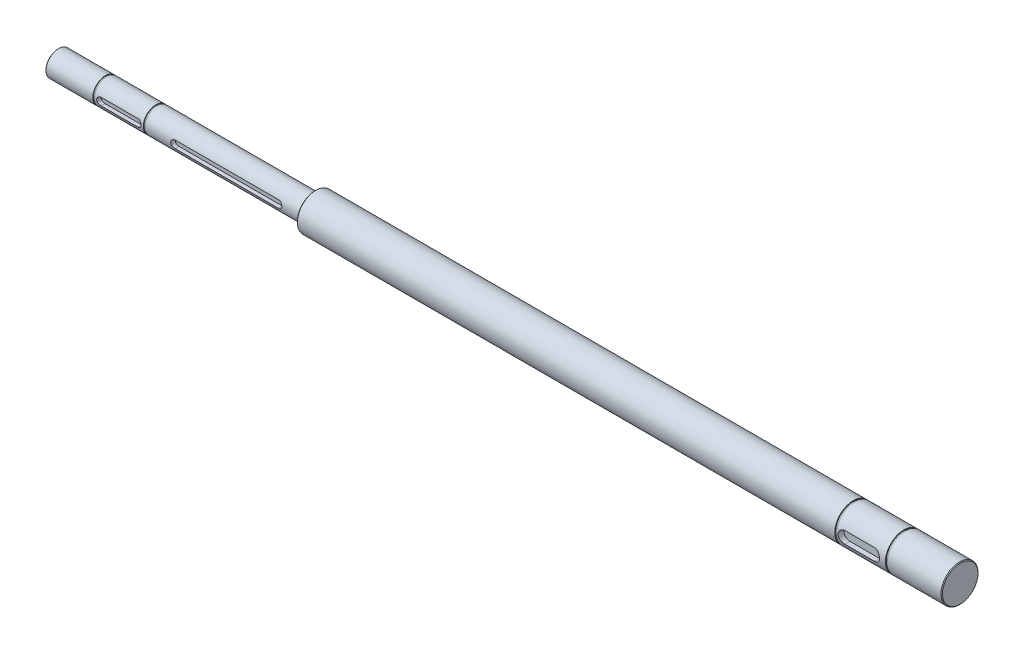
from build123d import *

# Parameters (mm, degrees)
SKETCH_2_R             = 12.5
EXTRUDE_1_DEPTH        = 304.5
SKETCH_3_OUTSIDE_W     = 149.006
SKETCH_3_OUTSIDE_H     = 149.006
SKETCH_3_OUTSIDE_R     = 8.5
CUT_EXTRUDE_1_DEPTH    = 173.5
CUT_EXTRUDE_2_DEPTH    = 3
CUT_EXTRUDE_3_DEPTH    = 4
CHAMFER_1_SIZE         = 0.5
CHAMFER_2_SIZE         = 0.3
SKETCH_8_W             = 1.2
SKETCH_8_H             = 0.55
PATTERN_LINEAR_2_COUNT = 2
PATTERN_LINEAR_2_PITCH = 34.2
SKETCH_9_W             = 1.1
SKETCH_9_H             = 0.4
PATTERN_LINEAR_3_COUNT = 2
PATTERN_LINEAR_3_PITCH = 34.1
FILLET_1_R             = 1.5


with BuildPart() as part:
    # 草图2 → 凸台-拉伸1 (new, symmetric)
    with BuildSketch(Plane(origin=(0, 0, 0), x_dir=(0, 0, -1), z_dir=(1, 0, 0))):
        Circle(SKETCH_2_R)
    extrude(amount=EXTRUDE_1_DEPTH, both=True)

    # 草图3 outside → 切除-拉伸1 (cut)
    with BuildSketch(Plane.ZY.offset(304.5)):
        Rectangle(SKETCH_3_OUTSIDE_W, SKETCH_3_OUTSIDE_H)
        Circle(SKETCH_3_OUTSIDE_R, mode=Mode.SUBTRACT)
    extrude(amount=-CUT_EXTRUDE_1_DEPTH, mode=Mode.SUBTRACT)

    # 草图5 → 切除-拉伸2 (cut)
    with BuildSketch(Plane.XY.offset(8.5)):
        with BuildLine():
            Line((-267.5, 2.5), (-242.5, 2.5))
            ThreePointArc((-242.5, 2.5), (-240, 0), (-242.5, -2.5))
            Line((-242.5, -2.5), (-267.5, -2.5))
            ThreePointArc((-267.5, -2.5), (-270, 0), (-267.5, 2.5))
        make_face()
        with BuildLine():
            Line((-217.5, 2.5), (-147.5, 2.5))
            ThreePointArc((-147.5, 2.5), (-145, 0), (-147.5, -2.5))
            Line((-147.5, -2.5), (-217.5, -2.5))
            ThreePointArc((-217.5, -2.5), (-220, 0), (-217.5, 2.5))
        make_face()
    extrude(amount=-CUT_EXTRUDE_2_DEPTH, mode=Mode.SUBTRACT)

    # 草图6 → 切除-拉伸3 (cut)
    with BuildSketch(Plane.XY.offset(12.5)):
        with BuildLine():
            Line((238.5, 4), (258.5, 4))
            ThreePointArc((258.5, 4), (262.5, 0), (258.5, -4))
            Line((258.5, -4), (238.5, -4))
            ThreePointArc((238.5, -4), (234.5, 0), (238.5, 4))
        make_face()
    extrude(amount=-CUT_EXTRUDE_3_DEPTH, mode=Mode.SUBTRACT)

    # 倒角1
    chamfer_1_edges = [part.edges().sort_by_distance(p)[0] for p in [
        (304.5, 0, 12.5),
        (-131, 0, 12.5),
    ]]
    chamfer(chamfer_1_edges, length=CHAMFER_1_SIZE)

    # 倒角2
    chamfer_2_edges = [part.edges().sort_by_distance(p)[0] for p in [
        (-304.5, 0, -8.5),
    ]]
    chamfer(chamfer_2_edges, length=CHAMFER_2_SIZE)

    # 草图8 → 切除-旋转2 (revolve, cut)
    with BuildSketch(Plane.XY, mode=Mode.PRIVATE) as cut_revolve_2_sk:
        with Locations((267.1, -12.225)):
            Rectangle(SKETCH_8_W, SKETCH_8_H)
    cut_revolve_2 = revolve(cut_revolve_2_sk.sketch.rotate(Axis((304.5, 0, 0), (-1, 0, 0)), 90), axis=Axis((304.5, 0, 0), (-1, 0, 0)), mode=Mode.SUBTRACT)

    # 阵列(线性)2: 切除-旋转2 ×2
    with Locations(*[(-i * PATTERN_LINEAR_2_PITCH, 0, 0) for i in range(1, PATTERN_LINEAR_2_COUNT)]):
        add(cut_revolve_2, mode=Mode.SUBTRACT)

    # 草图9 → 切除-旋转3 (revolve, cut)
    with BuildSketch(Plane.XY, mode=Mode.PRIVATE) as cut_revolve_3_sk:
        with Locations((-272.05, -8.3)):
            Rectangle(SKETCH_9_W, SKETCH_9_H)
    cut_revolve_3 = revolve(cut_revolve_3_sk.sketch.rotate(Axis((-131, 0, 0), (-1, 0, 0)), 270), axis=Axis((-131, 0, 0), (-1, 0, 0)), mode=Mode.SUBTRACT)

    # 阵列(线性)3: 切除-旋转3 ×2
    with Locations(*[(i * PATTERN_LINEAR_3_PITCH, 0, 0) for i in range(1, PATTERN_LINEAR_3_COUNT)]):
        add(cut_revolve_3, mode=Mode.SUBTRACT)

    # 圆角1
    fillet_1_edges = [part.edges().sort_by_distance(p)[0] for p in [
        (-131, 0, -8.5),
    ]]
    fillet(fillet_1_edges, radius=FILLET_1_R)


solid = part.part
